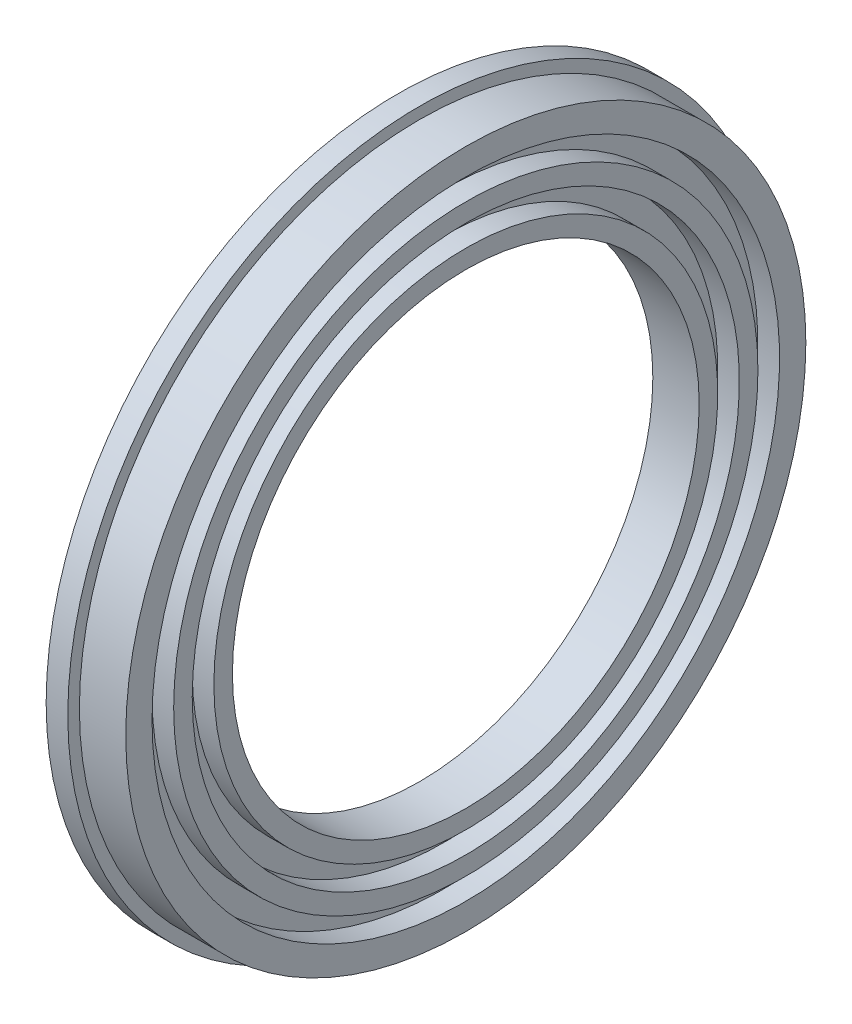
SolidWorks part; units mm, degrees
material "灰铸铁 HT150 "
ref_plane "Front Plane" through (0, 0, 0) normal (0, 0, 1) x (1, 0, 0)
ref_plane "Top Plane" through (0, 0, 0) normal (0, 1, 0) x (1, 0, 0)
ref_plane "Right Plane" through (0, 0, 0) normal (1, 0, 0) x (0, 0, -1)
sketch "Sketch1" plane through (0, 0, 0) normal (0, 1, 0) x (1, 0, 0)
  line L0 (0, 0) -> (170.742, 0) construction
  line L1 (0, 200) -> (0, 227.5)
  line L2 (0, 227.5) -> (14, 227.5)
  line L3 (14, 227.5) -> (14, 220)
  line L4 (14, 220) -> (44, 220)
  line L5 (44, 220) -> (44, 203)
  line L6 (44, 151) -> (14, 151)
  line L7 (14, 151) -> (14, 200)
  line L8 (14, 200) -> (0, 200)
  line L13 (44, 189) -> (44, 177)
  line L14 (44, 203) -> (30, 203)
  line L15 (44, 189) -> (30, 189)
  line L16 (30, 203) -> (30, 189)
  line L17 (44, 163) -> (44, 151)
  line L18 (44, 177) -> (30, 177)
  line L19 (44, 163) -> (30, 163)
  line L20 (30, 177) -> (30, 163)
  dimension "D1" = 151
  dimension "D2" = 200
  dimension "D3" = 227.5
  dimension "D4" = 14
  dimension "D5" = 44
  dimension "D6" = 220
  dimension "D7" = 203
  dimension "D8" = 14
  dimension "D9" = 14
  dimension "D10" = 163
  dimension "D11" = 177
  dimension "D12" = 189
revolve "Revolve1" add sketch "Sketch1" angle 360 about L0
fillet "Fillet1" radius 10 1 edges at (14, 0, 200)
